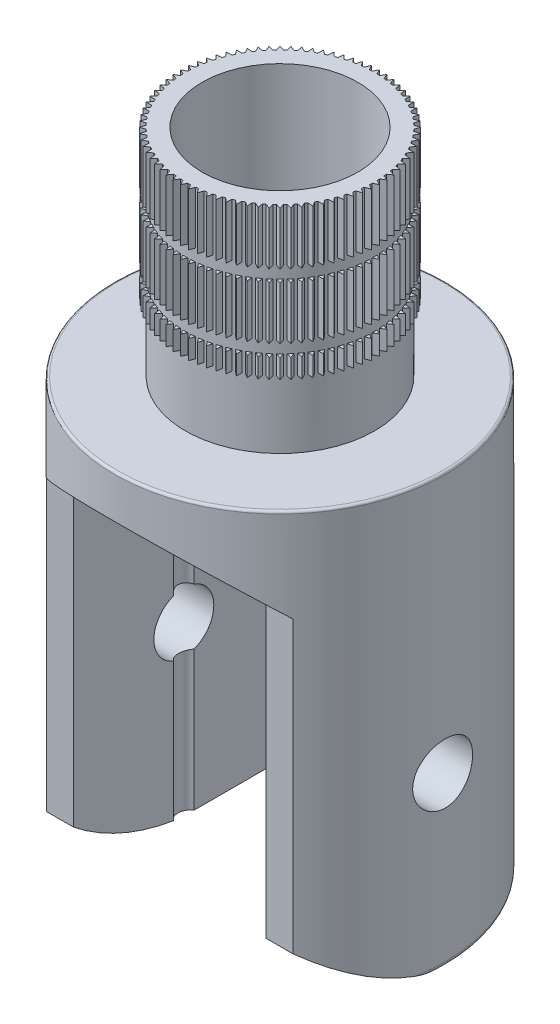
SolidWorks part; units mm, degrees
material "ABS"
ref_plane "Front Plane" through (0, 0, 0) normal (0, 0, 1) x (1, 0, 0)
ref_plane "Top Plane" through (0, 0, 0) normal (0, 1, 0) x (1, 0, 0)
ref_plane "Right Plane" through (0, 0, 0) normal (1, 0, 0) x (0, 0, -1)
sketch "Sketch1" plane through (0, 0, 0) normal (0, 0, 1) x (1, 0, 0)
  line L0 (0, 5.6839) -> (0, -2.2561) construction
  line L1 (0, 0) -> (-6.9, 0)
  line L2 (-6.9, 0) -> (-6.9, 17.9)
  line L3 (-6.9, 17.9) -> (-3.95, 17.9)
  line L5 (-3.95, 26.9) -> (0, 26.9)
  line L6 (0, 26.9) -> (0, 0)
  line L15 (-3.95, 17.9) -> (-3.95, 26.9)
  dimension "D1" = 7.9
  dimension "D2" = 13.8
  dimension "D3" = 17.9
  dimension "D4" = 9
revolve "Revolve1" add sketch "Sketch1" angle 360 about L0
sketch "Sketch3" plane through (0, 26.9, 0) normal (0, 1, 0) x (1, 0, 0)
  circle A3 centre (0, 0) radius 3.25
  dimension "D1" = 6.5
extrude "Cut-Extrude1" cut sketch "Sketch3" against normal offset from surface (8 mm away) 1 up to face at (-6.9, 17.9, 0)
sketch "Sketch5" plane through (0, 0, 0) normal (1, 0, 0) x (0, 0, -1)
  line L0 (-6.9, 16.1) -> (-4.6, 14)
  line L1 (6.9, 0) -> (6.9, 17.9) construction
  line L2 (-4.6, 14) -> (-4.6, 1.9)
  line L3 (-6.9, 16.1) -> (-6.9, 0)
  line L4 (-6.9, 0) -> (-0.1, 0)
  line L5 (-6.9, 0) -> (6.9, 0) construction
  line L7 (-6.9, 17.9) -> (-6.9, 0) construction
  line L8 (6.9, 0) -> (6.9, 17.9) construction
  line L11 (0, -1.8043) -> (0, 17.114) construction
  arc A1 (-4.6, 1.9) -> (-0.1, 0) centre (1.0194, 8.9301) ccw
  dimension "D2" = 9
  dimension "D3" = 11.5
  dimension "D5" = 12.1
  dimension "D6" = 7
  dimension "D1" = 16.1
  dimension "D4" = 14
extrude "Cut-Extrude3" cut sketch "Sketch5" against normal mid plane 15
sketch "Sketch4" plane through (0, 0, 0) normal (0, -1, 0) x (1, 0, 0)
  line L0 (0, 4.9187) -> (0, -5.3529) construction
  line L1 (4.0125, 7.3684) -> (4.0125, -4)
  line L2 (-4.0125, 7.3684) -> (4.0125, 7.3684)
  line L3 (-4.0125, 7.3684) -> (-4.0125, -4)
  line L4 (-4.0125, -4) -> (4.0125, -4)
  circle A1 centre (0, 0) radius 6.9 construction
  dimension "D1" = 8.025
  dimension "D2" = 2.9
extrude "Cut-Extrude2" cut sketch "Sketch4" against normal blind 14
sketch "Sketch8" plane through (0, 0, 0) normal (0, -1, 0) x (1, 0, 0)
  line L0 (-5.1631, 0) -> (5.8572, 0) construction
  line L1 (-4.0125, 0.1) -> (-4.0125, -4) construction
  line L2 (-4.0125, 0.4233) -> (-4.0125, -0.4233)
  line L3 (0, 0) -> (0, -2.2617) construction
  line L4 (4.0125, 0.4233) -> (4.0125, -0.4233)
  line L5 (-4.0125, 4.6) -> (-4.0125, -4) construction
  arc A0 (-4.0125, 0.4233) -> (-4.0125, -0.4233) centre (-3.7464, 0) ccw
  arc A1 (4.0125, 0.4233) -> (4.0125, -0.4233) centre (3.7464, 0) cw
  point P13 (-4.0125, 0)
  dimension "D1" = 0.5
extrude "Cut-Extrude6" cut sketch "Sketch8" against normal up to surface (14 mm away) up to face at (0, 14, 0.3)
sketch "Sketch9" plane through (0, 18.9, 0) normal (0, 1, 0) x (1, 0, 0)
  circle A0 centre (0, 0) radius 1.25
  dimension "D1" = 2.5
extrude "Cut-Extrude7" cut sketch "Sketch9" against normal up to surface (4.9 mm away)
sketch "Sketch10" plane through (0, 0, 0) normal (1, 0, 0) x (0, 0, -1)
  circle A0 centre (0, 7) radius 1.25
  dimension "D1" = 2.5
  dimension "D2" = 7
extrude "Cut-Extrude8" cut sketch "Sketch10" against normal blind 10 and the other way blind 10
fillet "Fillet1" radius 0.2 1 edges at (0, 0, -6.9)
sketch "Sketch11" plane through (0, 26.9, 0) normal (0, 1, 0) x (1, 0, 0)
  line L0 (0, 4.8735) -> (0, -5.1879) construction
  line L1 (-0.1, 3.9487) -> (0, 4.15)
  line L2 (0, 4.15) -> (0.1, 3.9487)
  circle A0 centre (0, 0) radius 3.95 construction
  arc A1 (0.1, 3.9487) -> (-0.1, 3.9487) centre (0, 0) ccw
  dimension "D1" = 0.2
  dimension "D2" = 0.2
extrude "Boss-Extrude1" add sketch "Sketch11" against normal blind 6.2
pattern_circular "CirPattern1" count 80 over 360 about axis through (0, 0, 0) along (0, 1, 0) of "Boss-Extrude1"
sketch "Sketch12" plane through (0, 0, 0) normal (1, 0, 0) x (0, 0, -1)
  line L0 (-4.15, 20.7) -> (-4.15, 26.9) construction
  line L1 (-4.15, 24.7) -> (-3.95, 24.7)
  line L2 (-4.15, 24.7) -> (-4.15, 24.2)
  line L3 (-4.15, 24.2) -> (-3.95, 24.2)
  line L4 (-3.95, 24.7) -> (-3.95, 24.2)
  line L5 (-4.15, 22) -> (-3.95, 22)
  line L6 (-4.15, 22) -> (-4.15, 21.5)
  line L7 (-4.15, 21.5) -> (-3.95, 21.5)
  line L8 (-3.95, 22) -> (-3.95, 21.5)
  dimension "D1" = 0.2
  dimension "D2" = 2.2
  dimension "D3" = 0.5
  dimension "D4" = 0.5
  dimension "D5" = 0.2
  dimension "D6" = 2.2
revolve "Cut-Revolve1" cut sketch "Sketch12" angle 360 about axis through (0, 8.7076, 0) along (0, 1, 0)
fillet "Fillet2" radius 0.1 1 edges at (-6.9, 17.9, 0)
